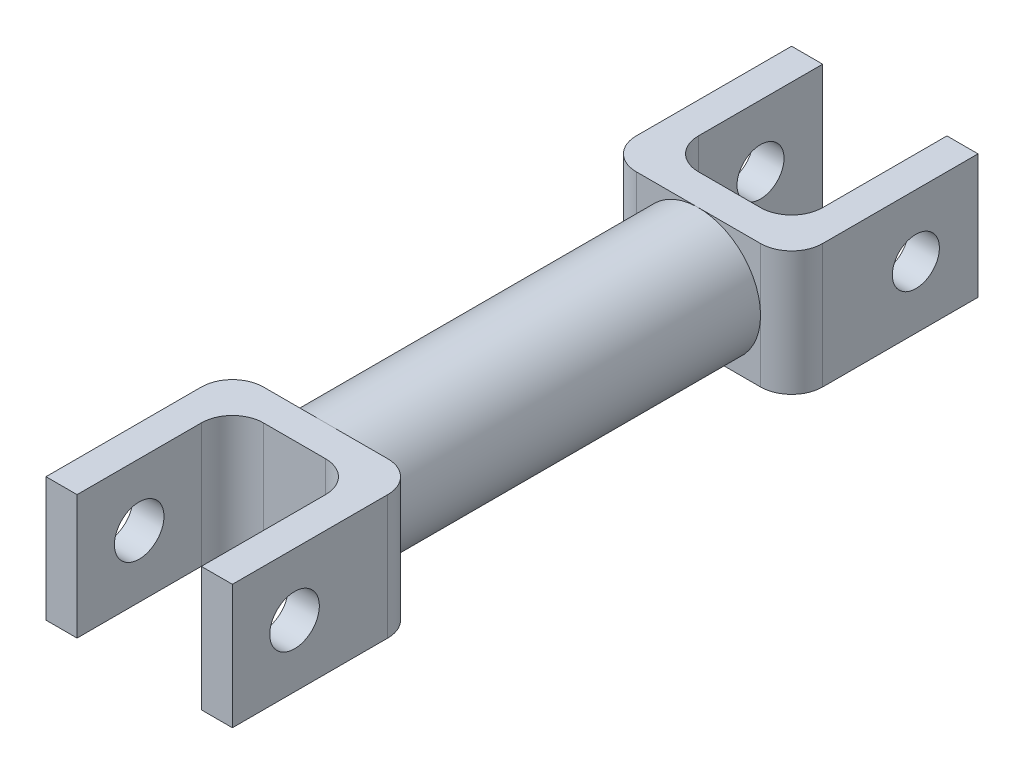
SolidWorks part; units mm, degrees
ref_plane "Front Plane" through (0, 0, 0) normal (0, 0, 1) x (1, 0, 0)
ref_plane "Top Plane" through (0, 0, 0) normal (0, 1, 0) x (1, 0, 0)
ref_plane "Right Plane" through (0, 0, 0) normal (1, 0, 0) x (0, 0, -1)
sketch "Sketch1" plane through (0, 0, 0) normal (0, 0, 1) x (1, 0, 0)
  circle A0 centre (0, 0) radius 10
  dimension "D1" = 20
extrude "Boss-Extrude1" add sketch "Sketch1" along normal blind 60
sketch "Sketch2" plane through (0, 0, 0) normal (0, 1, 0) x (1, 0, 0)
  line L0 (10, 0) -> (-10, 0) construction
  line L1 (-15, 30) -> (-10, 30)
  line L2 (-15, 30) -> (-15, 5)
  line L3 (-10, 0) -> (10, 0)
  line L4 (15, 30) -> (15, 5)
  line L5 (-10, 30) -> (-10, 10)
  line L6 (-5, 5) -> (5, 5)
  line L7 (10, 10) -> (10, 30)
  line L8 (10, 30) -> (15, 30)
  line L9 (-10, -30) -> (22.154, -30) construction
  line L10 (-10, 0) -> (-10, -60) construction
  line L11 (10, -90) -> (15, -90)
  line L12 (10, -70) -> (10, -90)
  line L13 (-5, -65) -> (5, -65)
  line L14 (-10, -90) -> (-10, -70)
  line L15 (15, -90) -> (15, -65)
  line L16 (-10, -60) -> (10, -60)
  line L17 (-15, -90) -> (-15, -65)
  line L18 (-15, -90) -> (-10, -90)
  arc A0 (-10, 10) -> (-5, 5) centre (-5, 10) ccw
  arc A1 (10, 0) -> (15, 5) centre (10, 5) ccw
  arc A2 (-15, 5) -> (-10, 0) centre (-10, 5) ccw
  arc A3 (5, 5) -> (10, 10) centre (5, 10) ccw
  arc A4 (5, -65) -> (10, -70) centre (5, -70) cw
  arc A5 (-15, -65) -> (-10, -60) centre (-10, -65) cw
  arc A6 (10, -60) -> (15, -65) centre (10, -65) cw
  arc A7 (-10, -70) -> (-5, -65) centre (-5, -70) cw
  point P15 (15, 0)
  point P40 (15, -60)
  dimension "D7" = 5
  dimension "D8" = 5
  dimension "D1" = 30
  dimension "D2" = 15
  dimension "D3" = 30
  dimension "D4" = 5
  dimension "D5" = 5
  dimension "D6" = 5
extrude "Boss-Extrude2" add sketch "Sketch2" along normal mid plane 20 separate body
sketch "Sketch3" plane through (-15, 0, 0) normal (-1, 0, 0) x (0, 0, 1)
  line L0 (90, 10) -> (90, -10) construction
  circle A0 centre (80, 0) radius 3.9893
  circle A1 centre (-20, 0) radius 3.7844
  dimension "D1" = 100
  dimension "D2" = 10
extrude "Cut-Extrude1" cut sketch "Sketch3" against normal through all
